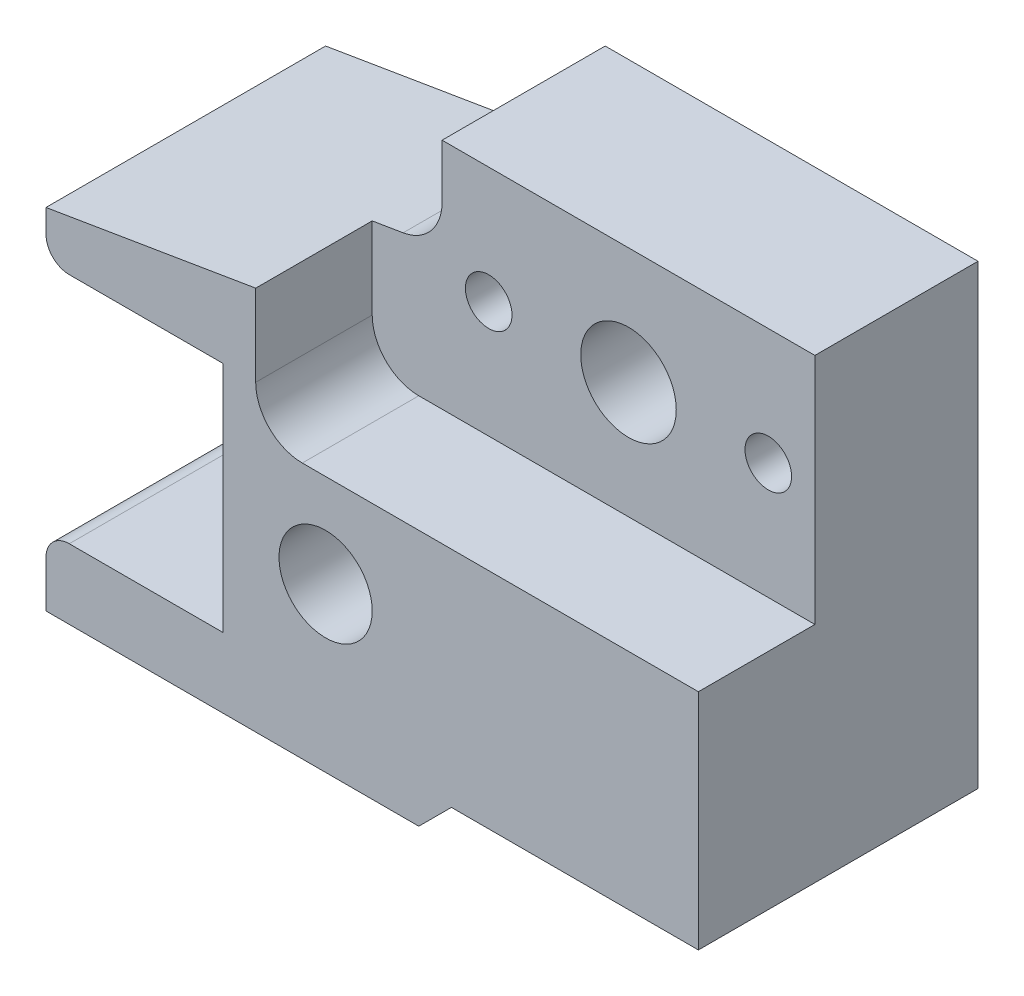
SolidWorks part; units mm, degrees
ref_plane "Front Plane" through (0, 0, 0) normal (0, 0, 1) x (1, 0, 0)
ref_plane "Top Plane" through (0, 0, 0) normal (0, 1, 0) x (1, 0, 0)
ref_plane "Right Plane" through (0, 0, 0) normal (1, 0, 0) x (0, 0, -1)
sketch "Sketch1" plane through (0, 0, 0) normal (0, 0, 1) x (1, 0, 0)
  line L1 (-7, 5.25) -> (7, 5.25)
  line L2 (-7, 5.25) -> (-7, -5.25)
  line L3 (-7, -5.25) -> (7, -5.25)
  line L4 (7, 5.25) -> (7, -5.25)
  line L5 (-7, 5.25) -> (7, -5.25) construction
  line L6 (-7, -5.25) -> (7, 5.25) construction
  point P0 (0, 0)
  dimension "D1" = 10.5
  dimension "D2" = 14
extrude "Boss-Extrude1" add sketch "Sketch1" along normal mid plane 6
sketch "Sketch2" plane through (0, 0, 3) normal (0, 0, 1) x (1, 0, 0)
  line L1 (7, 5.25) -> (-2.5, 5.25)
  line L2 (7, 5.25) -> (7, 0.25)
  line L3 (7, 0.25) -> (-2.5, 0.25)
  line L4 (-2.5, 5.25) -> (-2.5, 0.25)
  dimension "D1" = 5
  dimension "D2" = 9.5
extrude "Cut-Extrude1" cut sketch "Sketch2" against normal blind 2.5
sketch "Sketch3" plane through (0, 0, 3) normal (0, 0, 1) x (1, 0, 0)
  line L0 (-7, 5.25) -> (-1, 5.25)
  line L1 (7, 5.25) -> (-2.5, 5.25) construction
  line L2 (-1, 5.25) -> (-1, 3.25)
  line L3 (-1, 3.25) -> (-7, 2.25)
  line L4 (-7, 5.25) -> (-7, -5.25) construction
  line L5 (-7, 2.25) -> (-7, 5.25)
  line L6 (7, 0.25) -> (7, 5.25) construction
  line L7 (-7, -5.25) -> (7, -5.25) construction
  dimension "D1" = 8
  dimension "D2" = 7.5
  dimension "D3" = 2
extrude "Cut-Extrude2" cut sketch "Sketch3" against normal through all
fillet "Fillet1" radius 1 2 edges at (-2.5, 0.25, 1.75) (-1, 3.25, -1.25)
sketch "Sketch4" plane through (0, 0, 3) normal (0, 0, 1) x (1, 0, 0)
  line L0 (-7, 2.25) -> (-7, -5.25) construction
  line L1 (-7, -3.75) -> (-3.2, -3.75)
  line L2 (-7, -3.75) -> (-7, 1.25)
  line L3 (-7, 1.25) -> (-3.2, 1.25)
  line L4 (-3.2, -3.75) -> (-3.2, 1.25)
  line L5 (-7, -5.25) -> (7, -5.25) construction
  point P10 (-3.2, -3.75)
  dimension "D1" = 1.5
  dimension "D2" = 5
  dimension "D3" = 3.8
extrude "Cut-Extrude3" cut sketch "Sketch4" against normal through all
hole_wizard "M2.5 Tapped Hole1" positions "Sketch7" profile "Sketch6" tap size "M2.5" standard "Gb" end condition through all
sketch "Sketch7" plane through (0, 0, 0.5) normal (0, 0, 1) x (1, 0, 0)
  line L0 (7, 5.25) -> (-1, 5.25) construction
  line L1 (7, 0.25) -> (7, 5.25) construction
  point P0 (3, 2.75)
  dimension "D1" = 2.5
  dimension "D2" = 4
sketch "Sketch6" plane through (3, 2.75, 0.5) normal (1, 0, 0) x (0, -1, 0)
  line L0 (0, 0) -> (0, 3.5)
  line L1 (0, 3.5) -> (1.025, 3.5)
  line L2 (1.025, 3.5) -> (1.025, 0)
  line L5 (1.025, 0) -> (0, 0)
  line L11 (0, -6.35) -> (0, 107.95) construction
  dimension "通孔螺纹孔钻头直径" = 2.05
  dimension "通孔螺纹孔钻头深度" = 3.5
cosmetic thread "Hole Thread1" parameters "D2"=2.5
hole_wizard "Ø1.0 (1) Diameter Hole1" positions "Sketch9" profile "Sketch8" hole size "Ø1.0" standard "Gb" end condition through all
sketch "Sketch9" plane through (0, 0, 0.5) normal (0, 0, 1) x (1, 0, 0)
  line L0 (3, 2.75) -> (3, 6.1227) construction
  line L3 (3, 2.75) -> (7.6036, 2.75) construction
  point P0 (0, 2.75)
  point P2 (6, 2.75)
  dimension "D1" = 6
sketch "Sketch8" plane through (0, 2.75, 0.5) normal (1, 0, 0) x (0, -1, 0)
  line L0 (0, 0) -> (0, 3.5)
  line L1 (0, 3.5) -> (0.5, 3.5)
  line L2 (0.5, 3.5) -> (0.5, 0)
  line L5 (0.5, 0) -> (0, 0)
  line L11 (0, -6.35) -> (0, 107.95) construction
  dimension "通孔孔直径" = 1
  dimension "通孔孔深度" = 3.5
hole_wizard "Ø2.0 (2) Diameter Hole1" positions "Sketch12" profile "Sketch11" hole size "Ø2.0" standard "Gb" end condition through all
sketch "Sketch12" plane through (0, 0, 3) normal (0, 0, 1) x (1, 0, 0)
  line L0 (-7, -5.25) -> (7, -5.25) construction
  line L1 (7, -5.25) -> (7, 0.25) construction
  point P0 (-1, -1.75)
  dimension "D1" = 3.5
  dimension "D2" = 8
sketch "Sketch11" plane through (-1, -1.75, 3) normal (1, 0, 0) x (0, -1, 0)
  line L0 (0, 0) -> (0, 6)
  line L1 (0, 6) -> (1, 6)
  line L2 (1, 6) -> (1, 0)
  line L5 (1, 0) -> (0, 0)
  line L11 (0, -6.35) -> (0, 107.95) construction
  dimension "通孔孔直径" = 2
  dimension "通孔孔深度" = 6
sketch "Sketch15" plane through (0, 0, 3) normal (0, 0, 1) x (1, 0, 0)
  line L0 (7, -5.25) -> (1, -5.25)
  line L1 (-7, -5.25) -> (7, -5.25) construction
  line L2 (1, -5.25) -> (1.7, -4.55)
  line L3 (1.7, -4.55) -> (7, -4.55)
  line L4 (7, -5.25) -> (7, 0.25) construction
  line L5 (7, -4.55) -> (7, -5.25)
  dimension "D1" = 0.7
  dimension "D2" = 6
  dimension "D3" = 45
extrude "Cut-Extrude4" cut sketch "Sketch15" against normal through all
hole_wizard "Ø3.0 (3) Diameter Hole1" positions "Sketch17" profile "Sketch16" hole size "Ø3.0" standard "Gb"
sketch "Sketch17" plane through (0, -4.55, 0) normal (0, -1, 0) x (-1, 0, 0)
  line L0 (-7, 3) -> (-7, -3) construction
  point P0 (-4.2, 0)
  dimension "D1" = 2.8
sketch "Sketch16" plane through (4.2, -4.55, 0) normal (1, 0, 0) x (0, 0, -1)
  line L0 (0, 0) -> (0, 4.9013)
  line L1 (0, 4.9013) -> (1.5, 4)
  line L2 (1.5, 4) -> (1.5, 0)
  line L5 (1.5, 0) -> (0, 0)
  line L10 (0, 4.9013) -> (-1.5, 4) construction
  line L11 (0, -6.35) -> (0, 107.95) construction
  dimension "孔直径" = 3
  dimension "孔深度" = 4
  dimension "导头角度" = 118
fillet "Fillet2" radius 0.5 2 edges at (-7, 1.25, 0) (-7, -3.75, 0)
hole_wizard "M2.5 Tapped Hole2" positions "Sketch19" profile "Sketch18" tap size "M2.5" standard "Gb"
sketch "Sketch19" plane through (0, -5.25, 0) normal (0, -1, 0) x (-1, 0, 0)
  line L0 (2, -3) -> (2, 3) construction
  point P0 (1, 0)
  dimension "D1" = 1
sketch "Sketch18" plane through (-1, -5.25, 0) normal (1, 0, 0) x (0, 0, -1)
  line L0 (0, 0) -> (0, 4.6159)
  line L1 (0, 4.6159) -> (1.025, 4)
  line L2 (1.025, 4) -> (1.025, 0)
  line L5 (1.025, 0) -> (0, 0)
  line L10 (0, 4.6159) -> (-1.025, 4) construction
  line L11 (0, -6.35) -> (0, 107.95) construction
  dimension "螺纹孔钻头直径" = 2.05
  dimension "螺纹孔钻头深度" = 4
  dimension "导头角度" = 118
cosmetic thread "Hole Thread2" parameters "D1"=3, "D2"=2.5
